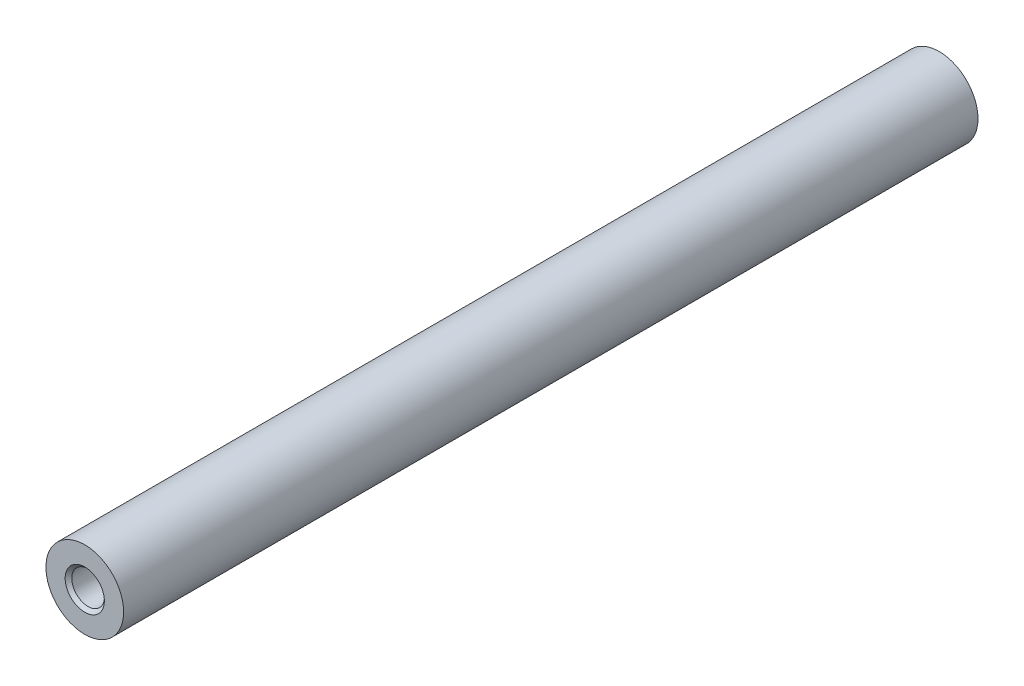
from build123d import *

# Parameters (mm, degrees)
SKETCH_1_R      = 5
EXTRUDE_1_DEPTH = 55


with BuildPart() as part:
    # 草图1 → 凸台-拉伸1 (new, symmetric)
    with BuildSketch(Plane.XY):
        Circle(SKETCH_1_R)
    extrude(amount=EXTRUDE_1_DEPTH, both=True)

    # 草图3 → M5x0.8 螺纹孔1 (revolve, cut)
    with BuildSketch(Plane(origin=(0, 0, 55), x_dir=(0, -1, 0), z_dir=(1, 0, 0))):
        Polygon((0, 0), (0, 13.6618073), (2.1, 12.4), (2.1, 0.425), (2.525, 0), align=None)
    m5x0_8_1 = revolve(axis=Axis((0, 0, 61.35), (0, 0, -1)), mode=Mode.SUBTRACT)

    # 镜向1: M5x0.8 螺纹孔1 across plane
    add(m5x0_8_1.mirror(Plane.XY), mode=Mode.SUBTRACT)


solid = part.part
